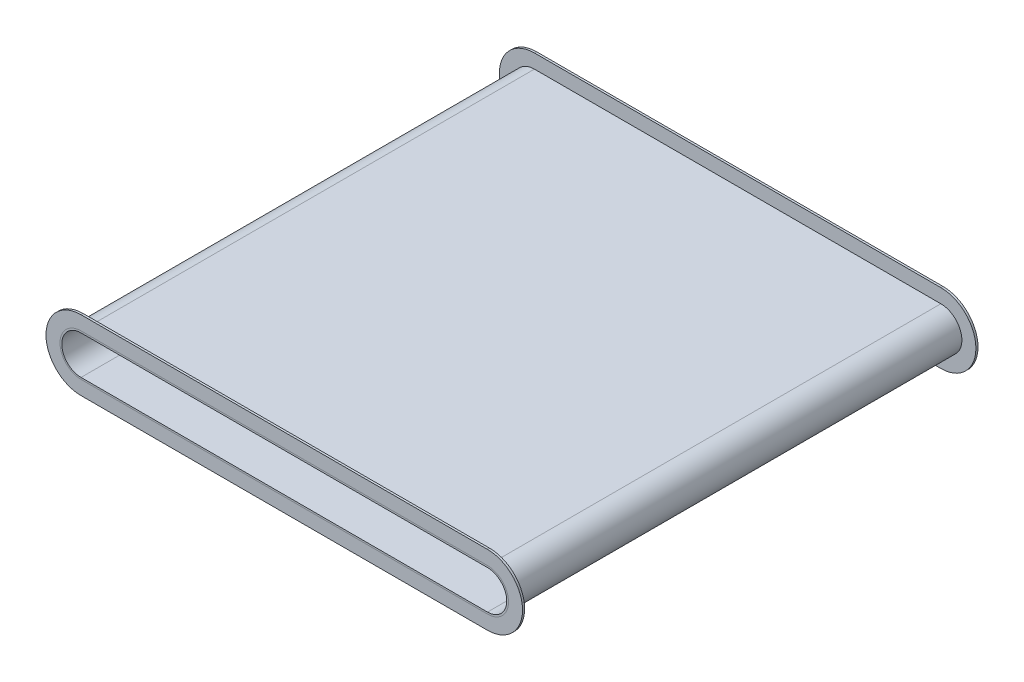
from build123d import *

# Parameters (mm, degrees)
BOSS_EXTRUDE1_DEPTH = 325
BOSS_EXTRUDE2_DEPTH = 3


with BuildPart() as part:
    # Sketch1 → Boss-Extrude1 (new, symmetric)
    with BuildSketch(Plane.XY):
        with BuildLine():
            Line((0, 30), (580, 30))
            ThreePointArc((580, 30), (610, 0), (580, -30))
            Line((580, -30), (0, -30))
            ThreePointArc((0, -30), (-30, 0), (0, 30))
        make_face()
        with BuildLine():
            Line((0, 27.5), (580, 27.5))
            ThreePointArc((580, 27.5), (607.5, 0), (580, -27.5))
            Line((580, -27.5), (0, -27.5))
            ThreePointArc((0, -27.5), (-27.5, 0), (0, 27.5))
        make_face(mode=Mode.SUBTRACT)
    extrude(amount=BOSS_EXTRUDE1_DEPTH, both=True)


with BuildPart() as body_2:
    # Sketch2 → Boss-Extrude2 (new body)
    with BuildSketch(Plane.XY.offset(325)):
        with BuildLine():
            Line((580, 50), (0, 50))
            ThreePointArc((0, 50), (-50, 0), (0, -50))
            Line((0, -50), (580, -50))
            ThreePointArc((580, -50), (630, 0), (580, 50))
        make_face()
        with BuildLine():
            Line((0, -30), (580, -30))
            ThreePointArc((580, -30), (610, 0), (580, 30))
            Line((580, 30), (0, 30))
            ThreePointArc((0, 30), (-30, 0), (0, -30))
        make_face(mode=Mode.SUBTRACT)
    extrude(amount=-BOSS_EXTRUDE2_DEPTH)


with BuildPart() as body_3:
    # Mirror1: mirrored copy
    add(body_2.part.mirror(Plane.XY))


solid = Compound([part.part, body_2.part, body_3.part])
